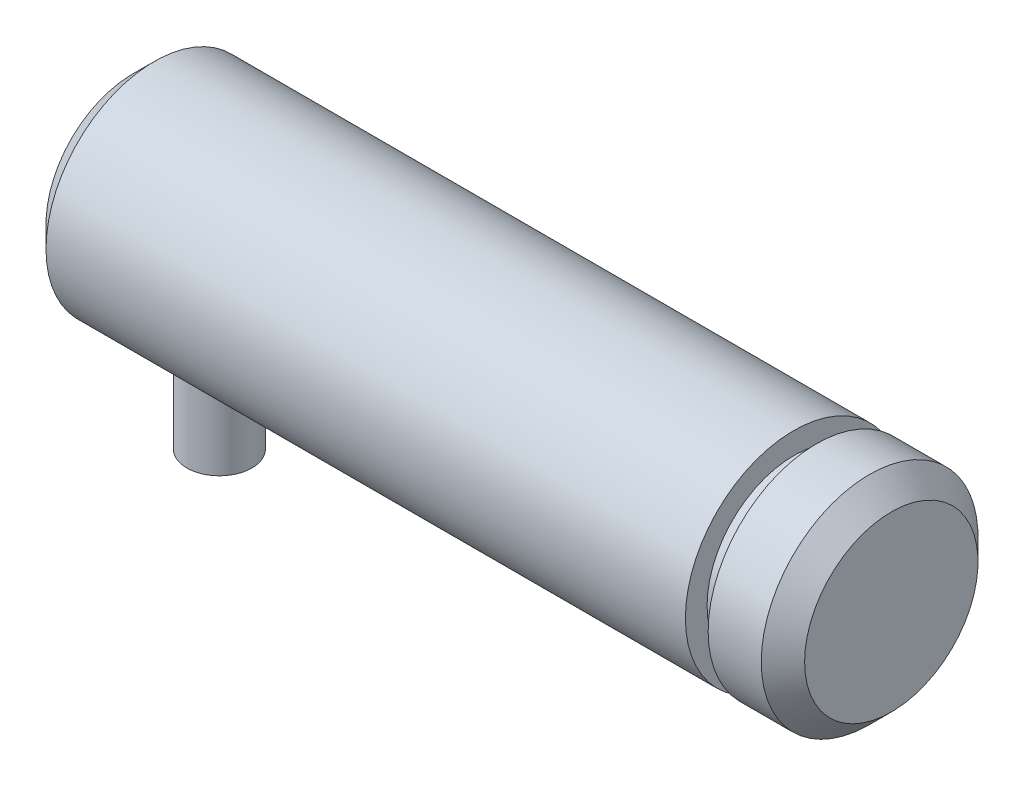
SolidWorks part; units mm, degrees
ref_plane "前视基准面" through (0, 0, 0) normal (0, 0, 1) x (1, 0, 0)
ref_plane "上视基准面" through (0, 0, 0) normal (0, 1, 0) x (1, 0, 0)
ref_plane "右视基准面" through (0, 0, 0) normal (1, 0, 0) x (0, 0, -1)
ref_plane "基准面4" through (0, 0, 0) normal (0, 0, -1) x (-1, 0, 0)
sketch "草图1" plane through (0, 0, 0) normal (0, 0, -1) x (-1, 0, 0)
  line L0 (-17.5, 5) -> (-17.5, 0)
  line L1 (-17.5, 0) -> (17.5, 0)
  line L2 (17.5, 0) -> (17.5, 5)
  line L3 (17.5, 5) -> (-13, 5)
  line L4 (-13, 5) -> (-13, 4)
  line L5 (-13, 4) -> (-14.05, 4)
  line L6 (-14.05, 4) -> (-14.05, 5)
  line L7 (-14.05, 5) -> (-17.5, 5)
  line L8 (-17.5, 0) -> (17.5, 0) construction
revolve "旋转1" add sketch "草图1" angle 360 about L8
ref_plane "基准面5" through (-13.5, 0, 0) normal (1, 0, 0) x (0, 0, -1)
sketch "草图2" plane through (-13.5, 0, 0) normal (1, 0, 0) x (0, 0, -1)
  line L0 (0, -9) -> (1.5, -9)
  line L1 (1.5, -9) -> (1.5, -4.7697)
  line L2 (1.5, -4.7697) -> (0, -4.7697)
  line L3 (0, -4.7697) -> (0, -9)
  line L4 (0, -4.7697) -> (0, -9) construction
revolve "旋转2" add sketch "草图2" angle 360 about L4
chamfer "倒角1" distance 1 angle 45 2 edges at (-17.5, 0, 5) (17.5, 0, 5)
